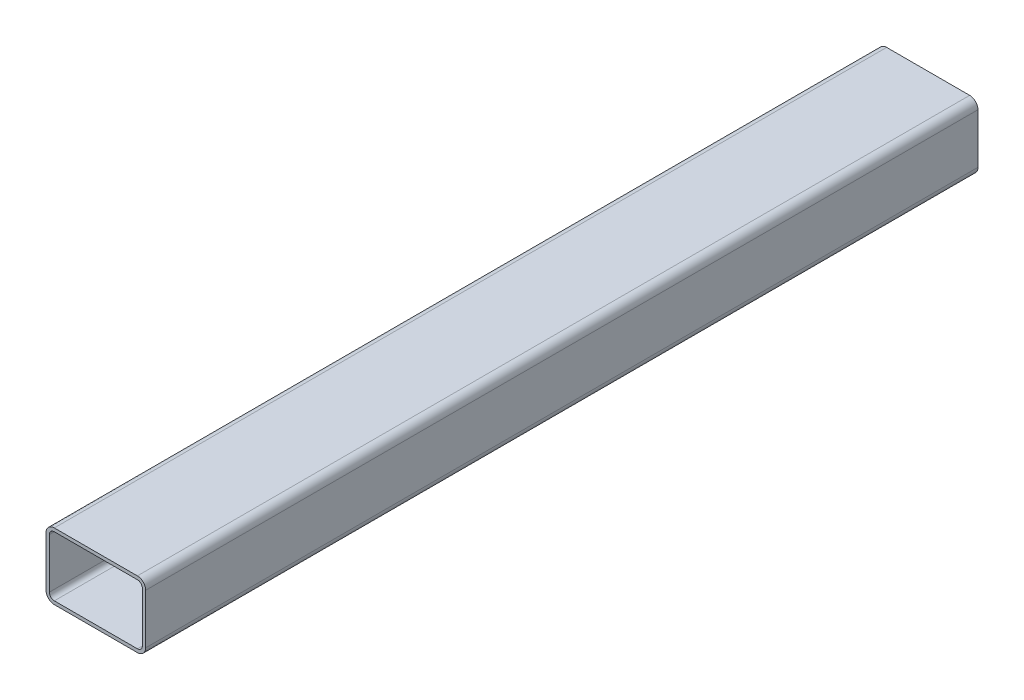
SolidWorks part; units mm, degrees
material "1023 碳钢板 (SS)"
ref_plane "Front Plane" through (0, 0, 0) normal (0, 0, 1) x (1, 0, 0)
ref_plane "Top Plane" through (0, 0, 0) normal (0, 1, 0) x (1, 0, 0)
ref_plane "Right Plane" through (0, 0, 0) normal (1, 0, 0) x (0, 0, -1)
sketch "Sketch1" plane through (0, 0, 0) normal (0, 0, 1) x (1, 0, 0)
  line L1 (60, 40) -> (-60, 40)
  line L2 (60, 40) -> (60, -40)
  line L3 (60, -40) -> (-60, -40)
  line L4 (-60, 40) -> (-60, -40)
  line L5 (60, 40) -> (-60, -40) construction
  line L6 (60, -40) -> (-60, 40) construction
  point P0 (0, 0)
  dimension "D1" = 120
  dimension "D2" = 80
extrude "Boss-Extrude1" add sketch "Sketch1" along normal blind 1002
fillet "Fillet1" radius 10 4 edges at (-60, -40, 501) (60, -40, 501) (60, 40, 501) (-60, 40, 501)
shell "Shell1" thickness 4
